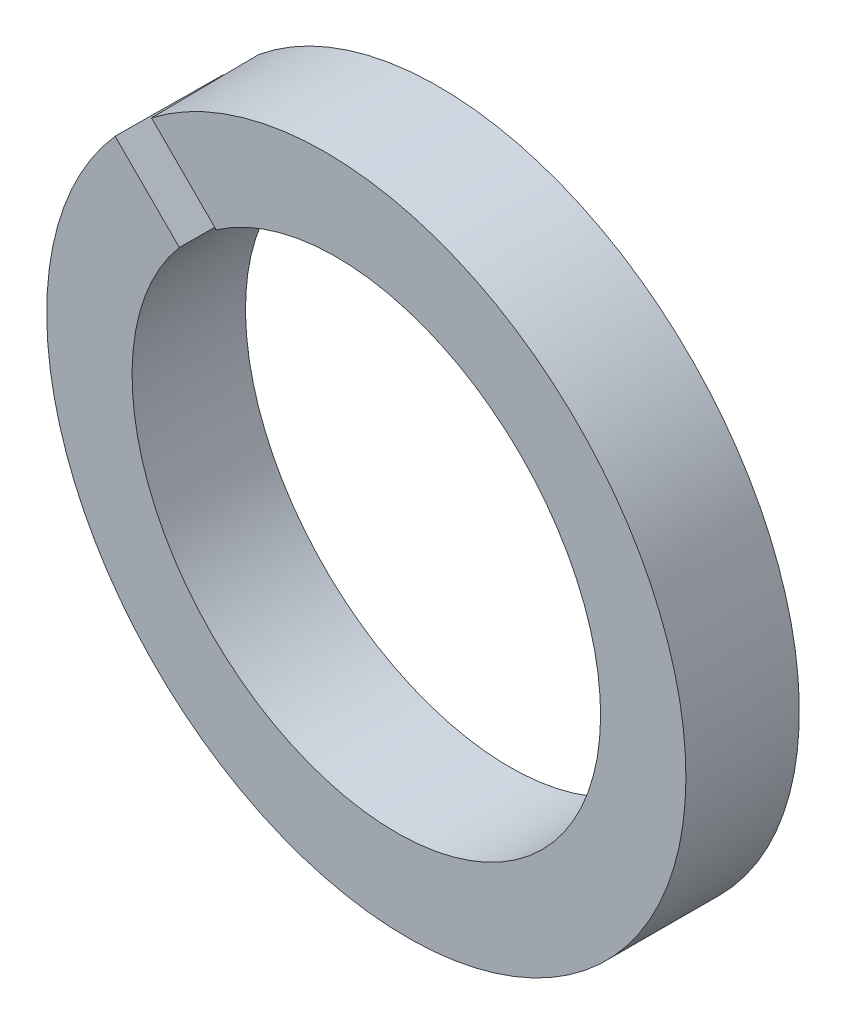
from build123d import *

# Parameters (mm, degrees)
BASE_EXTRUDE_DEPTH      = 0.001
BASE_EXTRUDE_DEPTH_BACK = 0.001
SKETCH6_W               = 4.71
SKETCH6_H               = 4.96
SKETCH8_R               = 15.00640628
SKETCH8_R_2             = 11
BOSS_EXTRUDE1_DEPTH     = 4.75
CUT_EXTRUDE1_DEPTH      = 23.559115412
CUT_EXTRUDE1_DEPTH_BACK = 23.559115412


with BuildPart() as part:
    # Sketch6 → Base-Extrude (new, two sides: drawn at the far end of the back side and taken through both)
    with BuildSketch(Plane(origin=(-7.071067812, 7.071067812, 5.25), x_dir=(0.05887808228355755, 0.05887808228355607, -0.9965273417489464), z_dir=(0.7046512409884902, 0.7046512409884782, 0.0832661824919251)).offset(-BASE_EXTRUDE_DEPTH_BACK)):
        with Locations((2.375, 2.5)):
            Rectangle(SKETCH6_W, SKETCH6_H)
    extrude(amount=BASE_EXTRUDE_DEPTH + BASE_EXTRUDE_DEPTH_BACK)

    # Sketch8 → Boss-Extrude1 (add)
    with BuildSketch(Plane(origin=(-0.306858937, -0.306858937, 5.193669853), x_dir=(0.9982651276202565, -0.00379884698167672, 0.05875630807770913), z_dir=(-0.05887808228355744, -0.05887808228355621, 0.9965273417489464))):
        with Locations(Location((0, 0, 0), (0, 0, 0.218036679))):
            Circle(SKETCH8_R)
        with Locations(Location((0, 0, 0), (0, 0, 0.218036679))):
            Circle(SKETCH8_R_2, mode=Mode.SUBTRACT)
    extrude(amount=-BOSS_EXTRUDE1_DEPTH)

    # Sketch9 → Cut-Extrude1 (cut, two sides: drawn at the far end of the back side and taken through both)
    with BuildSketch(Plane.XY.offset(-CUT_EXTRUDE1_DEPTH_BACK)):
        Polygon((-34.36706796, 36.134834913), (0.634717709, 1.133049244), (-1.133049244, -0.634717709), (-37.902601866, 36.134834913), align=None)
    extrude(amount=CUT_EXTRUDE1_DEPTH + CUT_EXTRUDE1_DEPTH_BACK, mode=Mode.SUBTRACT)


solid = part.part
